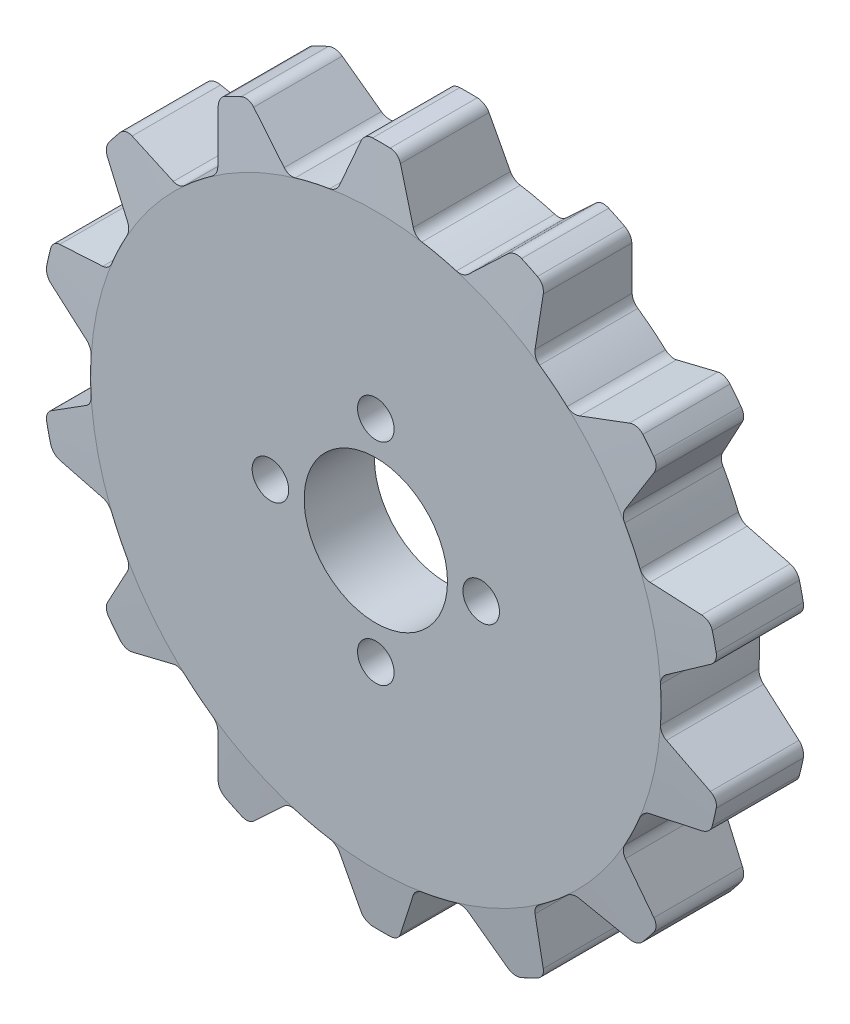
SolidWorks part; units mm, degrees
ref_plane "Front Plane" through (0, 0, 0) normal (0, 0, 1) x (1, 0, 0)
ref_plane "Top Plane" through (0, 0, 0) normal (0, 1, 0) x (1, 0, 0)
ref_plane "Right Plane" through (0, 0, 0) normal (1, 0, 0) x (0, 0, -1)
sketch "Sketch1" plane through (0, 0, 0) normal (0, 0, 1) x (1, 0, 0)
  circle A0 centre (0, 0) radius 101.5
  dimension "D1" = 203
extrude "Boss-Extrude1" add sketch "Sketch1" along normal blind 35
sketch "Sketch2" plane through (0, 0, 35) normal (0, 0, 1) x (1, 0, 0)
  line L2 (-7.0125, 118.7165) -> (-13.1074, 102.8529)
  line L3 (7.0125, 118.7165) -> (13.1074, 102.8529)
  arc A1 (3.1279, 121.4597) -> (-3.1279, 121.4597) centre (0, 0) ccw
  arc A2 (-16.4103, 100.1646) -> (-13.1074, 102.8529) centre (-17.1022, 104.3878) ccw
  arc A3 (16.4103, 100.1646) -> (13.1074, 102.8529) centre (17.1022, 104.3878) cw
  arc A4 (7.0125, 118.7165) -> (3.1279, 121.4597) centre (3.0177, 117.1817) ccw
  arc A5 (-3.1279, 121.4597) -> (-7.0125, 118.7165) centre (-3.0177, 117.1817) ccw
  arc A6 (16.4103, 100.1646) -> (-16.4103, 100.1646) centre (0, 0) ccw
  point P8 (-14, 100.5298)
  point P11 (14, 100.5298)
  point P14 (6, 121.3518)
  point P17 (-6, 121.3518)
  dimension "D2" = 243
  dimension "D5" = 4.2794
  dimension "D3" = 28
  dimension "D4" = 12
extrude "Boss-Extrude2" add sketch "Sketch2" against normal blind 35
pattern_circular "CirPattern1" count 14 over 360 about axis through (0, 0, 0) along (0, 0, 1) of "Boss-Extrude2"
sketch "Sketch3" plane through (0, 0, 0) normal (1, 0, 0) x (0, 0, -1)
  line L0 (-35, 121.4597) -> (-35, 101.4597)
  line L1 (-35, 118.7165) -> (-35, 102.8529) construction
  line L2 (-35, 101.4597) -> (-33, 121.4597)
  line L3 (0, 121.4597) -> (-35, 121.4597) construction
  line L4 (-33, 121.4597) -> (-33, 126.16)
  line L5 (-33, 126.16) -> (-35, 126.16)
  line L6 (-35, 126.16) -> (-35, 121.4597)
  line L7 (-17.5, 128.2641) -> (-17.5, 110.5204) construction
  line L8 (0, 126.16) -> (0, 121.4597)
  line L9 (-2, 126.16) -> (0, 126.16)
  line L10 (-2, 121.4597) -> (-2, 126.16)
  line L11 (0, 101.4597) -> (-2, 121.4597)
  line L12 (0, 121.4597) -> (0, 101.4597)
  dimension "D1" = 2
  dimension "D2" = 20
revolve "Cut-Revolve1" cut sketch "Sketch3" angle 360 about axis through (0, 0, 35) along (0, 0, -1)
sketch "Sketch4" plane through (0, 0, 35) normal (0, 0, 1) x (1, 0, 0)
  circle A0 centre (0, 0) radius 25.5
  point P18 (0, 0)
  dimension "D1" = 51
extrude "Cut-Extrude1" cut sketch "Sketch4" against normal through all
sketch "Sketch8" plane through (0, 0, 0) normal (0, 0, -1) x (-1, 0, 0)
  circle A1 centre (0, 0) radius 37.5 construction
  circle A2 centre (0, 37.5) radius 6.5
  circle A3 centre (37.5, 0) radius 6.5
  circle A4 centre (0, -37.5) radius 6.5
  circle A5 centre (-37.5, 0) radius 6.5
  point P15 (0, 0)
  dimension "D2" = 75
  dimension "D3" = 13
  dimension "D4" = 4
extrude "Cut-Extrude2" cut sketch "Sketch8" against normal through all
sketch "Sketch9" plane through (0, 0, 0) normal (0, 0, -1) x (-1, 0, 0)
  circle A0 centre (0, 0) radius 50.5
  dimension "D1" = 101
extrude "Cut-Extrude3" cut sketch "Sketch9" against normal blind 10
